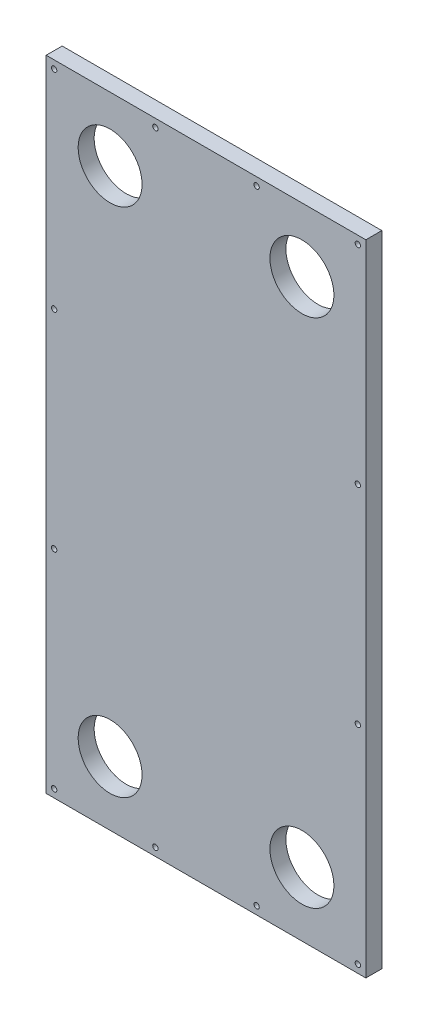
SolidWorks part; units mm, degrees
ref_plane "Front Plane" through (0, 0, 0) normal (0, 0, 1) x (1, 0, 0)
ref_plane "Top Plane" through (0, 0, 0) normal (0, 1, 0) x (1, 0, 0)
ref_plane "Right Plane" through (0, 0, 0) normal (1, 0, 0) x (0, 0, -1)
other "Configuration Table"
sketch "Sketch1" plane through (0, 0, 0) normal (0, 0, 1) x (1, 0, 0)
  line L1 (-300, -600) -> (300, -600)
  line L2 (-300, -600) -> (-300, 600)
  line L3 (-300, 600) -> (300, 600)
  line L4 (300, -600) -> (300, 600)
  line L5 (-300, -600) -> (300, 600) construction
  line L6 (-300, 600) -> (300, -600) construction
  point P0 (0, 0)
  dimension "D1" = 600
  dimension "D2" = 1200
extrude "Boss-Extrude1" add sketch "Sketch1" along normal blind 30
sketch "Sketch2" plane through (0, 0, 0) normal (0, 0, -1) x (-1, 0, 0)
  line L0 (0, 600) -> (0, -600) construction
  line L1 (-300, 600) -> (300, 600) construction
  line L2 (300, -600) -> (-300, -600) construction
  line L3 (-300, 0) -> (300, 0) construction
  line L4 (-300, -600) -> (-300, 600) construction
  line L5 (300, 600) -> (300, -600) construction
  circle A0 centre (-180, 480) radius 60
  circle A1 centre (180, 480) radius 60
  circle A2 centre (180, -480) radius 60
  circle A3 centre (-180, -480) radius 60
  dimension "D1" = 120
  dimension "D2" = 180
  dimension "D3" = 480
extrude "Cut-Extrude1" cut sketch "Sketch2" against normal blind 42
sketch "Sketch3" plane through (0, 0, 0) normal (0, 0, -1) x (-1, 0, 0)
  line L0 (-300, 600) -> (300, 600) construction
  line L1 (-300, -600) -> (-300, 600) construction
  circle A0 centre (-285, 585) radius 5
  dimension "D1" = 10
  dimension "D3" = 15
  dimension "D2" = 15
extrude "Cut-Extrude2" cut sketch "Sketch3" against normal blind 40
pattern_linear "LPattern1" count 4 spacing 390 along (0, -1, 0) of "Cut-Extrude2"
pattern_linear "LPattern2" count 2 spacing 570 along (-1, 0, 0) of "LPattern1", "Cut-Extrude2"
pattern_linear "LPattern3" count 3 spacing 190 along (-1, 0, 0) of "Cut-Extrude2"
pattern_linear "LPattern4" count 2 spacing 1170 along (0, -1, 0) of "LPattern3"
sketch "Sketch4" plane through (0, 0, 0) normal (0, 0, -1) x (-1, 0, 0)
  circle A0 centre (-285, 585) radius 10
  dimension "D1" = 20
extrude "Cut-Extrude3" cut sketch "Sketch4" against normal blind 15
pattern_linear "LPattern5" count 4 spacing 390 along (0, -1, 0) of "Cut-Extrude3"
pattern_linear "LPattern6" count 2 spacing 570 along (-1, 0, 0) of "LPattern5", "Cut-Extrude3"
pattern_linear "LPattern8" count 3 spacing 190 along (-1, 0, 0) of "Cut-Extrude3"
pattern_linear "LPattern9" count 2 spacing 1170 along (0, -1, 0) of "LPattern8"
